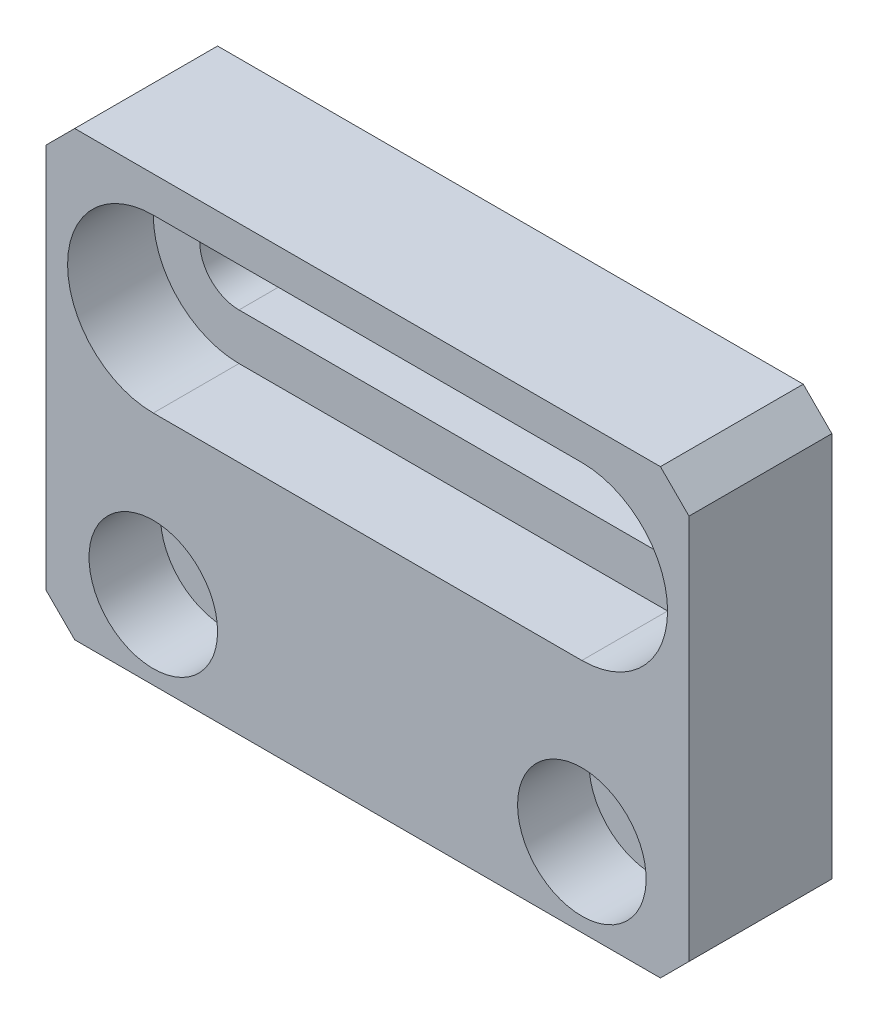
from build123d import *

# Parameters (mm, degrees)
SKETCH1_W           = 45
SKETCH1_H           = 31
BOSS_EXTRUDE1_DEPTH = 10
CUT_EXTRUDE1_DEPTH  = 13
SKETCH3_R           = 4.5
CUT_EXTRUDE2_DEPTH  = 5
SKETCH4_R           = 2.25
CUT_EXTRUDE3_DEPTH  = 14
CHAMFER1_SIZE       = 2
CUT_EXTRUDE4_DEPTH  = 6


with BuildPart() as part:
    # Sketch1 → Boss-Extrude1 (new body)
    with BuildSketch(Plane.XY):
        Rectangle(SKETCH1_W, SKETCH1_H)
    extrude(amount=BOSS_EXTRUDE1_DEPTH)

    # Sketch2 → Cut-Extrude1 (cut)
    with BuildSketch(Plane.XY.offset(10)):
        with BuildLine():
            Line((-15, 9.75), (15, 9.75))
            ThreePointArc((15, 9.75), (17.75, 7), (15, 4.25))
            Line((15, 4.25), (-15, 4.25))
            ThreePointArc((-15, 4.25), (-17.75, 7), (-15, 9.75))
        make_face()
    extrude(amount=-CUT_EXTRUDE1_DEPTH, mode=Mode.SUBTRACT)

    # Sketch3 → Cut-Extrude2 (cut)
    with BuildSketch(Plane.XY.offset(10)):
        with Locations((-15, -10)):
            Circle(SKETCH3_R)
        with Locations(Location((15, -10, 0), (0, 0, 180))):
            Circle(SKETCH3_R)
    extrude(amount=-CUT_EXTRUDE2_DEPTH, mode=Mode.SUBTRACT)

    # Sketch4 → Cut-Extrude3 (cut)
    with BuildSketch(Plane.XY.offset(10)):
        with Locations((-15, -10)):
            Circle(SKETCH4_R)
        with Locations((15, -10)):
            Circle(SKETCH4_R)
    extrude(amount=-CUT_EXTRUDE3_DEPTH, mode=Mode.SUBTRACT)

    # Chamfer1
    chamfer1_edges = [part.edges().sort_by_distance(p)[0] for p in [
        (22.5, -15.5, 5),
        (-22.5, -15.5, 5),
        (-22.5, 15.5, 5),
        (22.5, 15.5, 5),
    ]]
    chamfer(chamfer1_edges, length=CHAMFER1_SIZE)

    # Sketch5 → Cut-Extrude4 (cut)
    with BuildSketch(Plane.XY.offset(10)):
        with BuildLine():
            Line((-15, 13), (15, 13))
            ThreePointArc((15, 13), (21, 7), (15, 1))
            Line((15, 1), (-15, 1))
            ThreePointArc((-15, 1), (-21, 7), (-15, 13))
        make_face()
    extrude(amount=-CUT_EXTRUDE4_DEPTH, mode=Mode.SUBTRACT)


solid = part.part
